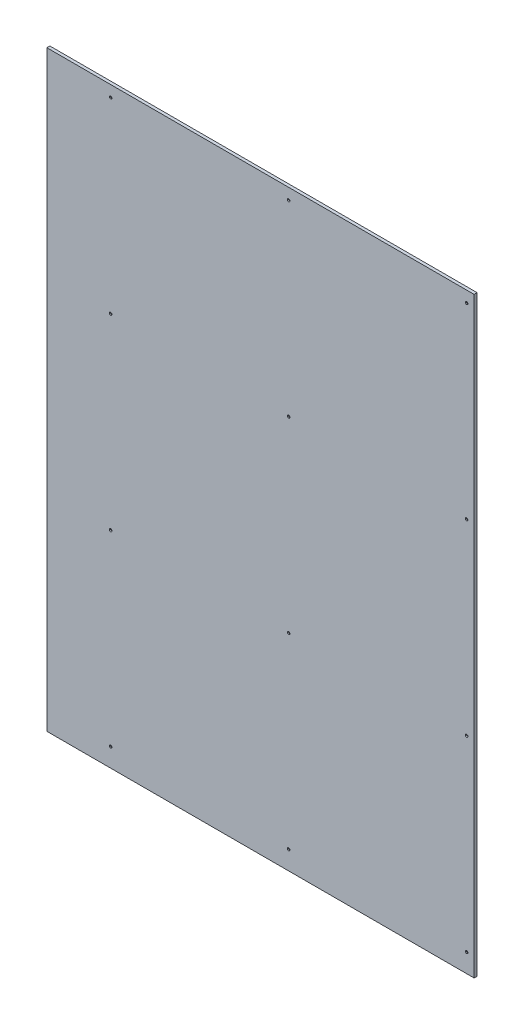
from build123d import *

# Parameters (mm, degrees)
SKETCH1_W                     = 1140
SKETCH1_H                     = 1580
BOSS_EXTRUDE1_DEPTH           = 8
SKETCH2_R                     = 3.5
CUT_EXTRUDE1_DEPTH            = 3
SKETCH3_R                     = 3.5
CUT_EXTRUDE2_DEPTH            = 5
CUT_EXTRUDE2_DRAFT            = 45
CUT_EXTRUDE2_PROFILE_2_DEPTH  = 5
CUT_EXTRUDE2_PROFILE_2_DRAFT  = 45
CUT_EXTRUDE2_PROFILE_3_DEPTH  = 5
CUT_EXTRUDE2_PROFILE_3_DRAFT  = 45
CUT_EXTRUDE2_PROFILE_4_DEPTH  = 5
CUT_EXTRUDE2_PROFILE_4_DRAFT  = 45
CUT_EXTRUDE2_PROFILE_5_DEPTH  = 5
CUT_EXTRUDE2_PROFILE_5_DRAFT  = 45
CUT_EXTRUDE2_PROFILE_6_DEPTH  = 5
CUT_EXTRUDE2_PROFILE_6_DRAFT  = 45
CUT_EXTRUDE2_PROFILE_7_DEPTH  = 5
CUT_EXTRUDE2_PROFILE_7_DRAFT  = 45
CUT_EXTRUDE2_PROFILE_8_DEPTH  = 5
CUT_EXTRUDE2_PROFILE_8_DRAFT  = 45
CUT_EXTRUDE2_PROFILE_9_DEPTH  = 5
CUT_EXTRUDE2_PROFILE_9_DRAFT  = 45
CUT_EXTRUDE2_PROFILE_10_DEPTH = 5
CUT_EXTRUDE2_PROFILE_10_DRAFT = 45
CUT_EXTRUDE2_PROFILE_11_DEPTH = 5
CUT_EXTRUDE2_PROFILE_11_DRAFT = 45
CUT_EXTRUDE2_PROFILE_12_DEPTH = 5
CUT_EXTRUDE2_PROFILE_12_DRAFT = 45


with BuildPart() as part:
    # Sketch1 → Boss-Extrude1 (new body)
    with BuildSketch(Plane.XY):
        Rectangle(SKETCH1_W, SKETCH1_H)
    extrude(amount=BOSS_EXTRUDE1_DEPTH)

    # Sketch2 → Cut-Extrude1 (cut)
    with BuildSketch(Plane.XY.offset(8)):
        with Locations((-400, -240)):
            Circle(SKETCH2_R)
        with Locations((75, -240)):
            Circle(SKETCH2_R)
        with Locations((550, -240)):
            Circle(SKETCH2_R)
        with Locations((-400, 260)):
            Circle(SKETCH2_R)
        with Locations((75, 260)):
            Circle(SKETCH2_R)
        with Locations((550, 260)):
            Circle(SKETCH2_R)
        with Locations((-400, 760)):
            Circle(SKETCH2_R)
        with Locations((75, 760)):
            Circle(SKETCH2_R)
        with Locations((550, 760)):
            Circle(SKETCH2_R)
        with Locations((-400, -740)):
            Circle(SKETCH2_R)
        with Locations((75, -740)):
            Circle(SKETCH2_R)
        with Locations((550, -740)):
            Circle(SKETCH2_R)
    extrude(amount=-CUT_EXTRUDE1_DEPTH, mode=Mode.SUBTRACT)


with BuildPart() as cut_extrude2_tool:
    # Sketch3 → Cut-Extrude2 (with draft: the straight prism first)
    with BuildSketch(Plane.XY.offset(5)):
        with Locations((550, -740)):
            Circle(SKETCH3_R)
    extrude(amount=-CUT_EXTRUDE2_DEPTH)
    # Cut-Extrude2: the draft: its side faces are tilted about the plane it starts from
    cut_extrude2_sides = [cut_extrude2_tool.faces().sort_by_distance(p)[0] for p in [
        (546.5, -740, 2.5),
    ]]
    draft(cut_extrude2_sides, Plane.XY.offset(5), CUT_EXTRUDE2_DRAFT)


with BuildPart() as part_1:
    add(part.part)

    # Cut-Extrude2: cut by cut_extrude2_tool
    add(cut_extrude2_tool.part, mode=Mode.SUBTRACT)


with BuildPart() as cut_extrude2_profile_2_tool:
    # Sketch3 → Cut-Extrude2 profile 2 (with draft: the straight prism first)
    with BuildSketch(Plane.XY.offset(5)):
        with Locations((75, -740)):
            Circle(SKETCH3_R)
    extrude(amount=-CUT_EXTRUDE2_PROFILE_2_DEPTH)
    # Cut-Extrude2 profile 2: the draft: its side faces are tilted about the plane it starts from
    cut_extrude2_profile_2_sides = [cut_extrude2_profile_2_tool.faces().sort_by_distance(p)[0] for p in [
        (71.5, -740, 2.5),
    ]]
    draft(cut_extrude2_profile_2_sides, Plane.XY.offset(5), CUT_EXTRUDE2_PROFILE_2_DRAFT)


with BuildPart() as part_2:
    add(part_1.part)

    # Cut-Extrude2 profile 2: cut by cut_extrude2_profile_2_tool
    add(cut_extrude2_profile_2_tool.part, mode=Mode.SUBTRACT)


with BuildPart() as cut_extrude2_profile_3_tool:
    # Sketch3 → Cut-Extrude2 profile 3 (with draft: the straight prism first)
    with BuildSketch(Plane.XY.offset(5)):
        with Locations((-400, -740)):
            Circle(SKETCH3_R)
    extrude(amount=-CUT_EXTRUDE2_PROFILE_3_DEPTH)
    # Cut-Extrude2 profile 3: the draft: its side faces are tilted about the plane it starts from
    cut_extrude2_profile_3_sides = [cut_extrude2_profile_3_tool.faces().sort_by_distance(p)[0] for p in [
        (-403.5, -740, 2.5),
    ]]
    draft(cut_extrude2_profile_3_sides, Plane.XY.offset(5), CUT_EXTRUDE2_PROFILE_3_DRAFT)


with BuildPart() as part_3:
    add(part_2.part)

    # Cut-Extrude2 profile 3: cut by cut_extrude2_profile_3_tool
    add(cut_extrude2_profile_3_tool.part, mode=Mode.SUBTRACT)


with BuildPart() as cut_extrude2_profile_4_tool:
    # Sketch3 → Cut-Extrude2 profile 4 (with draft: the straight prism first)
    with BuildSketch(Plane.XY.offset(5)):
        with Locations((-400, -240)):
            Circle(SKETCH3_R)
    extrude(amount=-CUT_EXTRUDE2_PROFILE_4_DEPTH)
    # Cut-Extrude2 profile 4: the draft: its side faces are tilted about the plane it starts from
    cut_extrude2_profile_4_sides = [cut_extrude2_profile_4_tool.faces().sort_by_distance(p)[0] for p in [
        (-403.5, -240, 2.5),
    ]]
    draft(cut_extrude2_profile_4_sides, Plane.XY.offset(5), CUT_EXTRUDE2_PROFILE_4_DRAFT)


with BuildPart() as part_4:
    add(part_3.part)

    # Cut-Extrude2 profile 4: cut by cut_extrude2_profile_4_tool
    add(cut_extrude2_profile_4_tool.part, mode=Mode.SUBTRACT)


with BuildPart() as cut_extrude2_profile_5_tool:
    # Sketch3 → Cut-Extrude2 profile 5 (with draft: the straight prism first)
    with BuildSketch(Plane.XY.offset(5)):
        with Locations((75, -240)):
            Circle(SKETCH3_R)
    extrude(amount=-CUT_EXTRUDE2_PROFILE_5_DEPTH)
    # Cut-Extrude2 profile 5: the draft: its side faces are tilted about the plane it starts from
    cut_extrude2_profile_5_sides = [cut_extrude2_profile_5_tool.faces().sort_by_distance(p)[0] for p in [
        (71.5, -240, 2.5),
    ]]
    draft(cut_extrude2_profile_5_sides, Plane.XY.offset(5), CUT_EXTRUDE2_PROFILE_5_DRAFT)


with BuildPart() as part_5:
    add(part_4.part)

    # Cut-Extrude2 profile 5: cut by cut_extrude2_profile_5_tool
    add(cut_extrude2_profile_5_tool.part, mode=Mode.SUBTRACT)


with BuildPart() as cut_extrude2_profile_6_tool:
    # Sketch3 → Cut-Extrude2 profile 6 (with draft: the straight prism first)
    with BuildSketch(Plane.XY.offset(5)):
        with Locations((550, -240)):
            Circle(SKETCH3_R)
    extrude(amount=-CUT_EXTRUDE2_PROFILE_6_DEPTH)
    # Cut-Extrude2 profile 6: the draft: its side faces are tilted about the plane it starts from
    cut_extrude2_profile_6_sides = [cut_extrude2_profile_6_tool.faces().sort_by_distance(p)[0] for p in [
        (546.5, -240, 2.5),
    ]]
    draft(cut_extrude2_profile_6_sides, Plane.XY.offset(5), CUT_EXTRUDE2_PROFILE_6_DRAFT)


with BuildPart() as part_6:
    add(part_5.part)

    # Cut-Extrude2 profile 6: cut by cut_extrude2_profile_6_tool
    add(cut_extrude2_profile_6_tool.part, mode=Mode.SUBTRACT)


with BuildPart() as cut_extrude2_profile_7_tool:
    # Sketch3 → Cut-Extrude2 profile 7 (with draft: the straight prism first)
    with BuildSketch(Plane.XY.offset(5)):
        with Locations((550, 260)):
            Circle(SKETCH3_R)
    extrude(amount=-CUT_EXTRUDE2_PROFILE_7_DEPTH)
    # Cut-Extrude2 profile 7: the draft: its side faces are tilted about the plane it starts from
    cut_extrude2_profile_7_sides = [cut_extrude2_profile_7_tool.faces().sort_by_distance(p)[0] for p in [
        (546.5, 260, 2.5),
    ]]
    draft(cut_extrude2_profile_7_sides, Plane.XY.offset(5), CUT_EXTRUDE2_PROFILE_7_DRAFT)


with BuildPart() as part_7:
    add(part_6.part)

    # Cut-Extrude2 profile 7: cut by cut_extrude2_profile_7_tool
    add(cut_extrude2_profile_7_tool.part, mode=Mode.SUBTRACT)


with BuildPart() as cut_extrude2_profile_8_tool:
    # Sketch3 → Cut-Extrude2 profile 8 (with draft: the straight prism first)
    with BuildSketch(Plane.XY.offset(5)):
        with Locations((75, 260)):
            Circle(SKETCH3_R)
    extrude(amount=-CUT_EXTRUDE2_PROFILE_8_DEPTH)
    # Cut-Extrude2 profile 8: the draft: its side faces are tilted about the plane it starts from
    cut_extrude2_profile_8_sides = [cut_extrude2_profile_8_tool.faces().sort_by_distance(p)[0] for p in [
        (71.5, 260, 2.5),
    ]]
    draft(cut_extrude2_profile_8_sides, Plane.XY.offset(5), CUT_EXTRUDE2_PROFILE_8_DRAFT)


with BuildPart() as part_8:
    add(part_7.part)

    # Cut-Extrude2 profile 8: cut by cut_extrude2_profile_8_tool
    add(cut_extrude2_profile_8_tool.part, mode=Mode.SUBTRACT)


with BuildPart() as cut_extrude2_profile_9_tool:
    # Sketch3 → Cut-Extrude2 profile 9 (with draft: the straight prism first)
    with BuildSketch(Plane.XY.offset(5)):
        with Locations((-400, 260)):
            Circle(SKETCH3_R)
    extrude(amount=-CUT_EXTRUDE2_PROFILE_9_DEPTH)
    # Cut-Extrude2 profile 9: the draft: its side faces are tilted about the plane it starts from
    cut_extrude2_profile_9_sides = [cut_extrude2_profile_9_tool.faces().sort_by_distance(p)[0] for p in [
        (-403.5, 260, 2.5),
    ]]
    draft(cut_extrude2_profile_9_sides, Plane.XY.offset(5), CUT_EXTRUDE2_PROFILE_9_DRAFT)


with BuildPart() as part_9:
    add(part_8.part)

    # Cut-Extrude2 profile 9: cut by cut_extrude2_profile_9_tool
    add(cut_extrude2_profile_9_tool.part, mode=Mode.SUBTRACT)


with BuildPart() as cut_extrude2_profile_10_tool:
    # Sketch3 → Cut-Extrude2 profile 10 (with draft: the straight prism first)
    with BuildSketch(Plane.XY.offset(5)):
        with Locations((550, 760)):
            Circle(SKETCH3_R)
    extrude(amount=-CUT_EXTRUDE2_PROFILE_10_DEPTH)
    # Cut-Extrude2 profile 10: the draft: its side faces are tilted about the plane it starts from
    cut_extrude2_profile_10_sides = [cut_extrude2_profile_10_tool.faces().sort_by_distance(p)[0] for p in [
        (546.5, 760, 2.5),
    ]]
    draft(cut_extrude2_profile_10_sides, Plane.XY.offset(5), CUT_EXTRUDE2_PROFILE_10_DRAFT)


with BuildPart() as part_10:
    add(part_9.part)

    # Cut-Extrude2 profile 10: cut by cut_extrude2_profile_10_tool
    add(cut_extrude2_profile_10_tool.part, mode=Mode.SUBTRACT)


with BuildPart() as cut_extrude2_profile_11_tool:
    # Sketch3 → Cut-Extrude2 profile 11 (with draft: the straight prism first)
    with BuildSketch(Plane.XY.offset(5)):
        with Locations((75, 760)):
            Circle(SKETCH3_R)
    extrude(amount=-CUT_EXTRUDE2_PROFILE_11_DEPTH)
    # Cut-Extrude2 profile 11: the draft: its side faces are tilted about the plane it starts from
    cut_extrude2_profile_11_sides = [cut_extrude2_profile_11_tool.faces().sort_by_distance(p)[0] for p in [
        (71.5, 760, 2.5),
    ]]
    draft(cut_extrude2_profile_11_sides, Plane.XY.offset(5), CUT_EXTRUDE2_PROFILE_11_DRAFT)


with BuildPart() as part_11:
    add(part_10.part)

    # Cut-Extrude2 profile 11: cut by cut_extrude2_profile_11_tool
    add(cut_extrude2_profile_11_tool.part, mode=Mode.SUBTRACT)


with BuildPart() as cut_extrude2_profile_12_tool:
    # Sketch3 → Cut-Extrude2 profile 12 (with draft: the straight prism first)
    with BuildSketch(Plane.XY.offset(5)):
        with Locations((-400, 760)):
            Circle(SKETCH3_R)
    extrude(amount=-CUT_EXTRUDE2_PROFILE_12_DEPTH)
    # Cut-Extrude2 profile 12: the draft: its side faces are tilted about the plane it starts from
    cut_extrude2_profile_12_sides = [cut_extrude2_profile_12_tool.faces().sort_by_distance(p)[0] for p in [
        (-403.5, 760, 2.5),
    ]]
    draft(cut_extrude2_profile_12_sides, Plane.XY.offset(5), CUT_EXTRUDE2_PROFILE_12_DRAFT)


with BuildPart() as part_12:
    add(part_11.part)

    # Cut-Extrude2 profile 12: cut by cut_extrude2_profile_12_tool
    add(cut_extrude2_profile_12_tool.part, mode=Mode.SUBTRACT)


solid = part_12.part
